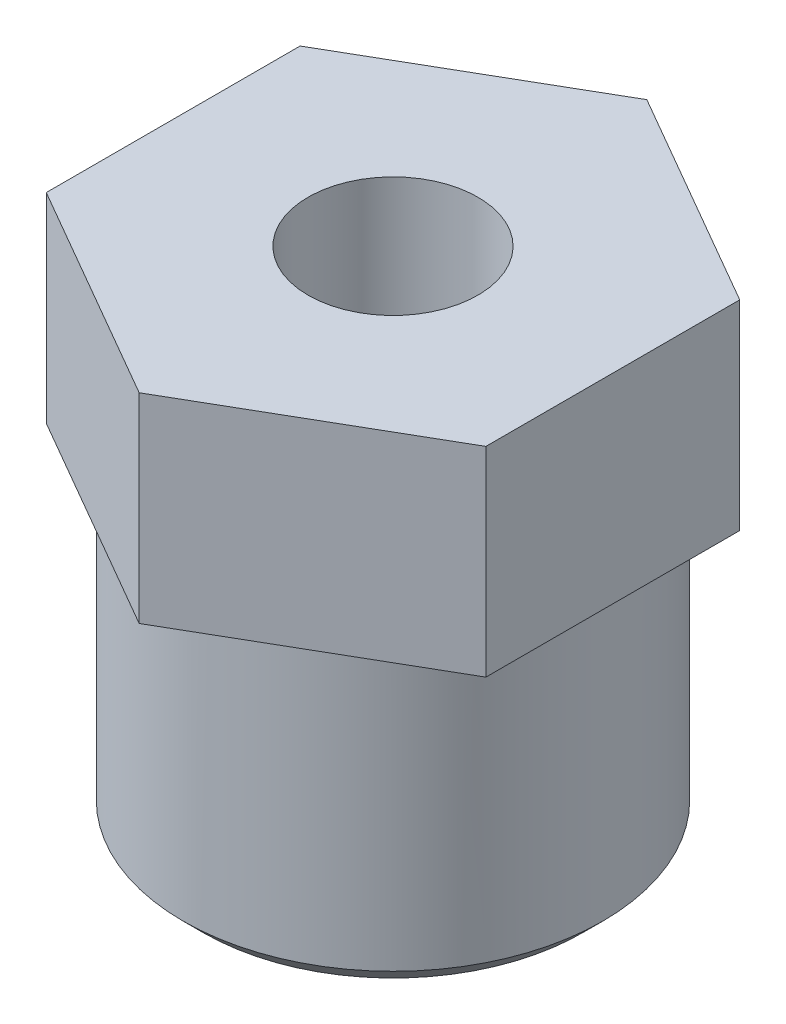
SolidWorks part; units mm, degrees
material "AISI 304"
ref_plane "Front Plane" through (0, 0, 0) normal (0, 0, 1) x (1, 0, 0)
ref_plane "Top Plane" through (0, 0, 0) normal (0, 1, 0) x (1, 0, 0)
ref_plane "Right Plane" through (0, 0, 0) normal (1, 0, 0) x (0, 0, -1)
sketch "Sketch1" plane through (0, 0, 0) normal (0, 1, 0) x (1, 0, 0)
  line L1 (11, -6.3509) -> (11, 6.3509)
  line L2 (11, 6.3509) -> (0, 12.7017)
  line L3 (0, 12.7017) -> (-11, 6.3509)
  line L4 (-11, 6.3509) -> (-11, -6.3509)
  line L5 (-11, -6.3509) -> (0, -12.7017)
  line L6 (0, -12.7017) -> (11, -6.3509)
  circle A0 centre (0, 0) radius 11 construction
  dimension "D1" = 22
extrude "Boss-Extrude1" add sketch "Sketch1" along normal blind 25
sketch "Sketch3" plane through (0, 0, 0) normal (0, -1, 0) x (1, 0, 0)
  circle A0 centre (0, 0) radius 10.5
  dimension "D1" = 21
extrude "Cut-Extrude1" cut sketch "Sketch3" against normal offset from surface (15 mm away) 10 flip side to cut up to face at (0, 25, 0)
cosmetic thread "Cosmetic Thread1" parameters "D2"=18.631
chamfer "Chamfer1" distance 1 angle 45 1 edges at (0, 0, -10.5)
sketch "Sketch9" plane through (0, 25, 0) normal (0, 1, 0) x (1, 0, 0)
  point P0 (0, 0)
hole_wizard "M10 Tapped Hole1" positions "3DSketch1" profile "Sketch10" tap size "M10" standard "GB" end condition through all
sketch3d "3DSketch1"
  point P0 (0, 25, 0)
sketch "Sketch10" plane through (0, 25, 0) normal (1, 0, 0) x (0, 0, 1)
  line L0 (0, 0) -> (0, 25)
  line L1 (0, 25) -> (4.25, 25)
  line L2 (4.25, 25) -> (4.25, 0)
  line L5 (4.25, 0) -> (0, 0)
  line L11 (0, -6.35) -> (0, 107.95) construction
  dimension "通孔螺纹孔钻头直径" = 8.5
  dimension "通孔螺纹孔钻头深度" = 25
cosmetic thread "Hole Cosmetic Thread1" parameters "D2"=10
